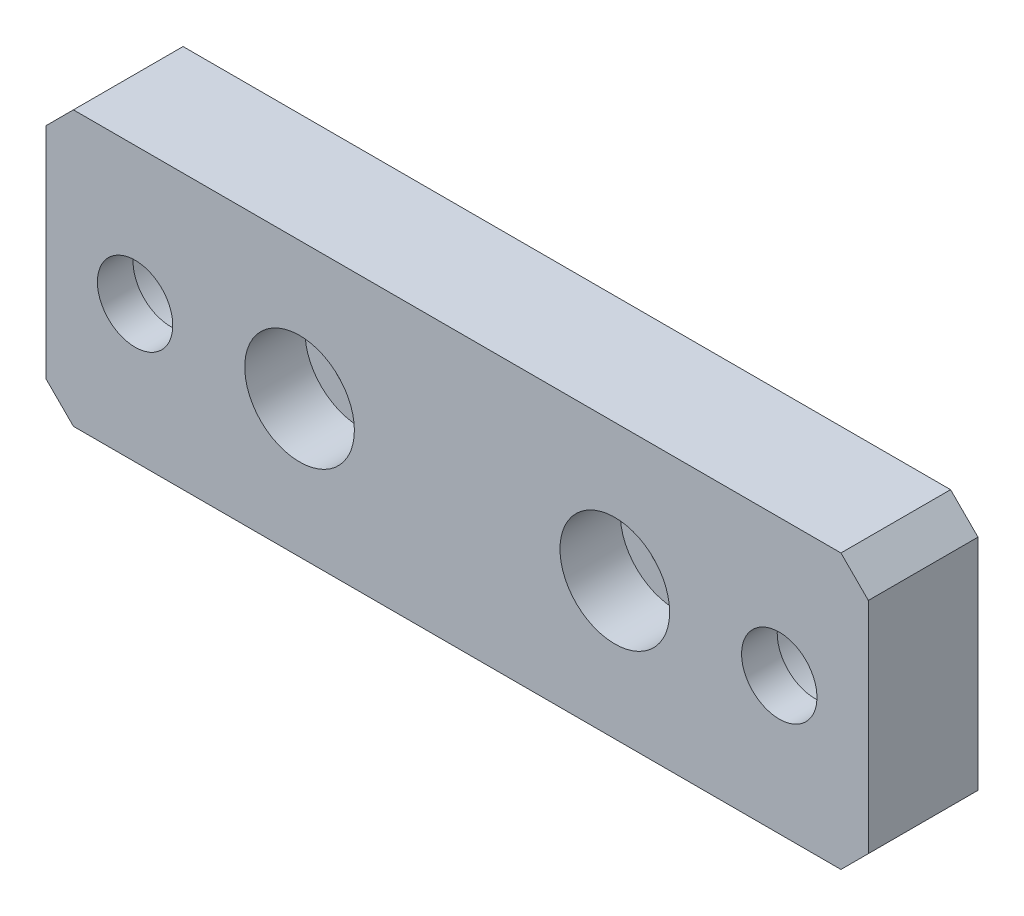
from build123d import *

# Parameters (mm, degrees)
SKETCH1_W                                           = 60
SKETCH1_H                                           = 20
BOSS_EXTRUDE1_DEPTH                                 = 8
CBORE_FOR_M4_HEX_SOCKET_HEAD_CAP_SCREW2_D           = 4.5
CBORE_FOR_M4_HEX_SOCKET_HEAD_CAP_SCREW2_CBORE_D     = 8
CBORE_FOR_M4_HEX_SOCKET_HEAD_CAP_SCREW2_CBORE_DEPTH = 4.4
CBORE_FOR_M5_HEX_SOCKET_HEAD_CAP_SCREW1_D           = 5.5
CBORE_FOR_M5_HEX_SOCKET_HEAD_CAP_SCREW1_CBORE_D     = 10
CBORE_FOR_M5_HEX_SOCKET_HEAD_CAP_SCREW1_CBORE_DEPTH = 5.4
CHAMFER1_SIZE                                       = 2


with BuildPart() as part:
    # Sketch1 → Boss-Extrude1 (new body)
    with BuildSketch(Plane.XY):
        with Locations((30, 10)):
            Rectangle(SKETCH1_W, SKETCH1_H)
    extrude(amount=BOSS_EXTRUDE1_DEPTH)

    # CBORE for M4 Hex Socket Head Cap Screw2 (through all)
    with Locations(Plane.XY.offset(8)):
        with Locations((41.5, 10), (18.5, 10)):
            CounterBoreHole(CBORE_FOR_M4_HEX_SOCKET_HEAD_CAP_SCREW2_D / 2, CBORE_FOR_M4_HEX_SOCKET_HEAD_CAP_SCREW2_CBORE_D / 2, CBORE_FOR_M4_HEX_SOCKET_HEAD_CAP_SCREW2_CBORE_DEPTH)

    # CBORE for M5 Hex Socket Head Cap Screw1 (through all)
    with Locations(Plane(origin=(0, 0, 0), x_dir=(1, 0, 0), z_dir=(0, 0, -1))):
        with Locations((53.5, -10), (6.5, -10)):
            CounterBoreHole(CBORE_FOR_M5_HEX_SOCKET_HEAD_CAP_SCREW1_D / 2, CBORE_FOR_M5_HEX_SOCKET_HEAD_CAP_SCREW1_CBORE_D / 2, CBORE_FOR_M5_HEX_SOCKET_HEAD_CAP_SCREW1_CBORE_DEPTH)

    # Chamfer1
    chamfer1_edges = [part.edges().sort_by_distance(p)[0] for p in [
        (0, 20, 4),
        (60, 20, 4),
        (60, 0, 4),
        (0, 0, 4),
    ]]
    chamfer(chamfer1_edges, length=CHAMFER1_SIZE)


solid = part.part
